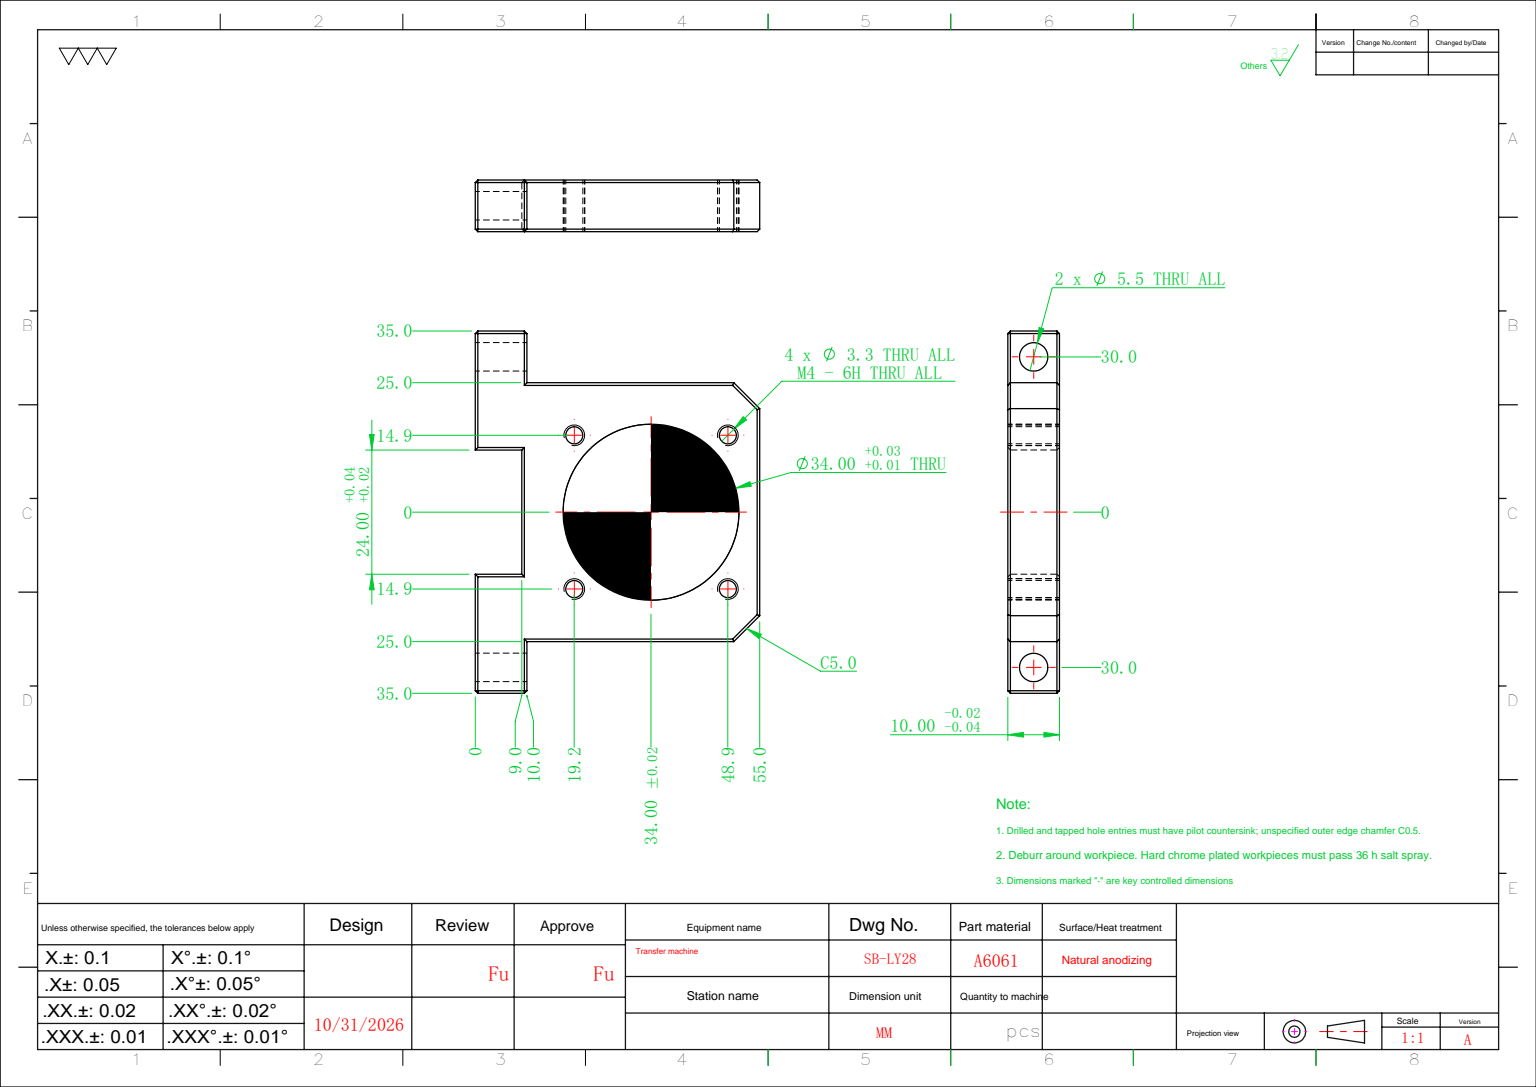
from build123d import *

# Parameters (mm, degrees)
SKETCH_1_W              = 70
SKETCH_1_H              = 55
EXTRUDE_1_DEPTH         = 10
SKETCH_2_W              = 10
SKETCH_2_H              = 45
CUT_EXTRUDE_1_DEPTH     = 46.620718977
SKETCH_3_R              = 17
CUT_EXTRUDE_2_DEPTH     = 46.620718977
HOLE_WIZARD_M4_2_D      = 3.3
HOLE_WIZARD_5_5_5_5_1_D = 5.5
CHAMFER_1_SIZE          = 5
SKETCH_12_W             = 24
SKETCH_12_H             = 9
CUT_EXTRUDE_3_DEPTH     = 46.620718977
CHAMFER_2_SIZE          = 0.5


with BuildPart() as part:
    # 草图1 → 凸台-拉伸1 (new body)
    with BuildSketch(Plane.XY):
        Rectangle(SKETCH_1_W, SKETCH_1_H)
    extrude(amount=EXTRUDE_1_DEPTH)

    # 草图2 → 切除-拉伸1 (cut, through all)
    with BuildSketch(Plane.XY.offset(10)):
        with Locations((-30, -5)):
            Rectangle(SKETCH_2_W, SKETCH_2_H)
        with Locations((30, -5)):
            Rectangle(SKETCH_2_W, SKETCH_2_H)
    extrude(amount=-CUT_EXTRUDE_1_DEPTH, mode=Mode.SUBTRACT)

    # 草图3 → 切除-拉伸2 (cut, through all)
    with BuildSketch(Plane(origin=(0, 0, 0), x_dir=(-1, 0, 0), z_dir=(0, 0, -1))):
        with Locations((0, -6.5)):
            Circle(SKETCH_3_R)
    extrude(amount=-CUT_EXTRUDE_2_DEPTH, mode=Mode.SUBTRACT)

    # M4 螺纹孔2 (through all)
    with Locations(Plane.XY.offset(10)):
        with Locations((14.85, -21.35), (-14.85, -21.35), (-14.85, 8.35), (14.85, 8.35)):
            Hole(HOLE_WIZARD_M4_2_D / 2)

    # Ø5.5 (5.5) 直径孔1 (through all)
    with Locations(Plane(origin=(0, 17.5, 0), x_dir=(-1, 0, 0), z_dir=(0, -1, 0))):
        with Locations((-30, -5), (30, -5)):
            Hole(HOLE_WIZARD_5_5_5_5_1_D / 2)

    # 倒角1
    chamfer_1_edges = [part.edges().sort_by_distance(p)[0] for p in [
        (-25, -27.5, 5),
        (25, -27.5, 5),
    ]]
    chamfer(chamfer_1_edges, length=CHAMFER_1_SIZE)

    # 草图12 → 切除-拉伸3 (cut, through all)
    with BuildSketch(Plane.XY.offset(10)):
        with Locations((0, 23)):
            Rectangle(SKETCH_12_W, SKETCH_12_H)
    extrude(amount=-CUT_EXTRUDE_3_DEPTH, mode=Mode.SUBTRACT)

    # 倒角2
    chamfer_2_edges = [part.edges().sort_by_distance(p)[0] for p in [
        (-35, 22.5, 10),
        (0, 18.5, 10),
        (12, 23, 10),
        (-30, 17.5, 0),
        (-35, 17.5, 5),
        (-30, 17.5, 10),
        (35, 22.5, 0),
        (35, 22.5, 10),
        (25, -2.5, 0),
        (30, 17.5, 0),
        (35, 17.5, 5),
        (30, 17.5, 10),
        (25, -2.5, 10),
        (-35, 22.5, 0),
        (23.5, 27.5, 0),
        (23.5, 27.5, 10),
        (-35, 27.5, 5),
        (35, 27.5, 5),
        (-25, -2.5, 10),
        (-25, -2.5, 0),
        (0, -27.5, 10),
        (22.5, -25, 10),
        (-22.5, -25, 10),
        (0, -27.5, 0),
        (22.5, -25, 0),
        (-22.5, -25, 0),
        (-23.5, 27.5, 0),
        (-23.5, 27.5, 10),
        (-12, 23, 0),
        (12, 23, 0),
        (0, 18.5, 0),
        (-12, 23, 10),
    ]]
    chamfer(chamfer_2_edges, length=CHAMFER_2_SIZE)


solid = part.part
